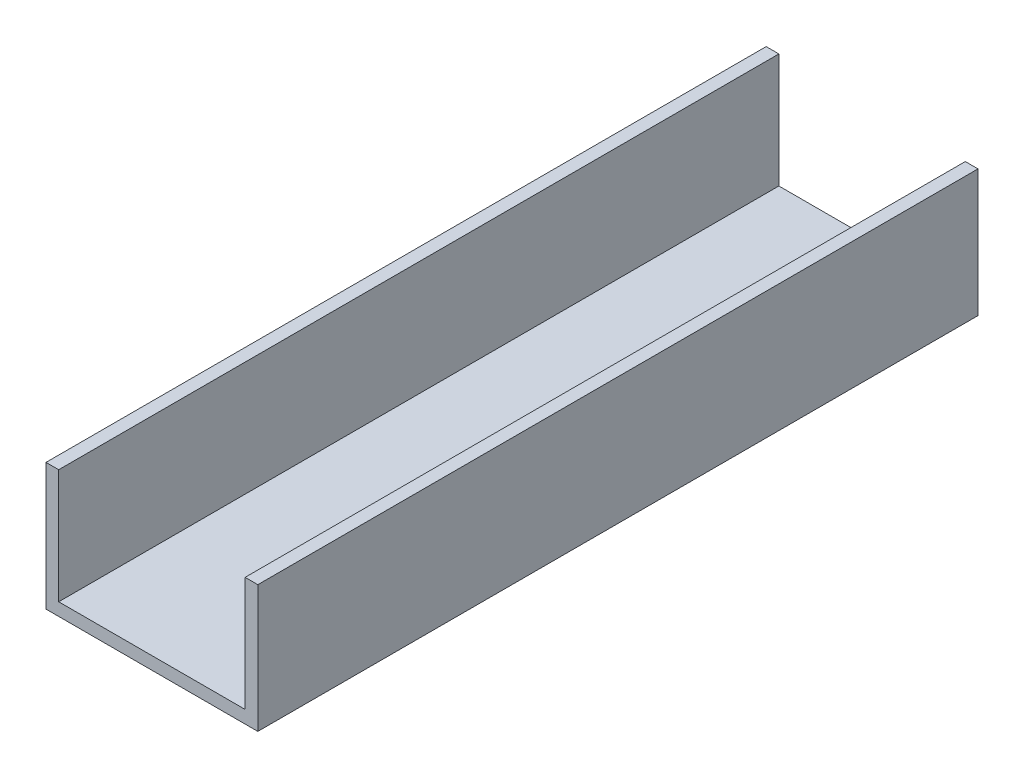
from build123d import *

# Parameters (mm, degrees)
EXTRUDE_1_DEPTH     = 340
CUT_EXTRUDE_1_DEPTH = 170


with BuildPart() as part:
    # 草图1 → 凸台-拉伸1 (new body)
    with BuildSketch(Plane.XY):
        Polygon((0, 0), (0, 30), (3, 30), (3, 3), (47, 3), (47, 30), (50, 30), (50, 0), align=None)
    extrude(amount=EXTRUDE_1_DEPTH)

    # 草图2 → 切除-拉伸1 (cut)
    with BuildSketch(Plane.XY.offset(340)):
        Polygon((0, 0), (50, 0), (50, 30), (47, 30), (47, 3), (3, 3), (3, 30), (0, 30), align=None)
    extrude(amount=-CUT_EXTRUDE_1_DEPTH, mode=Mode.SUBTRACT)


solid = part.part
